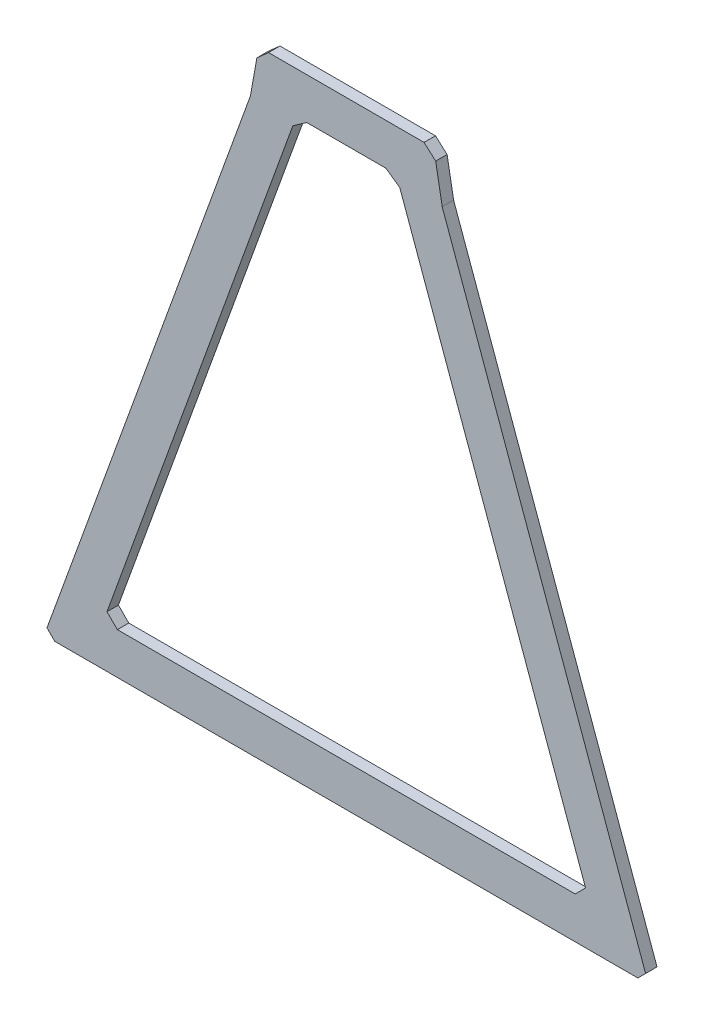
from build123d import *

# Parameters (mm, degrees)
BOSS_EXTRUDE1_DEPTH = 14


with BuildPart() as part:
    # Sketch1 → Boss-Extrude1 (new body)
    with BuildSketch(Plane.XY):
        Polygon((-95.25, 755.65), (0, 755.65), (95.25, 755.65), (109.5375, 742.95), (117.475, 698.5), (366.7125, 9.525), (357.1875, 0), (0, 0), (-357.1875, 0), (-366.7125, 9.525), (-117.475, 698.5), (-109.5375, 742.95), align=None)
        Polygon((-280.465202582, 50.8), (280.465202582, 50.8), (293.165202582, 63.5), (65.476347176, 692.907409213), (48.4561012, 704.85), (-48.4561012, 704.85), (-65.476347176, 692.907409213), (-293.165202582, 63.5), align=None, mode=Mode.SUBTRACT)
    extrude(amount=BOSS_EXTRUDE1_DEPTH)


solid = part.part
